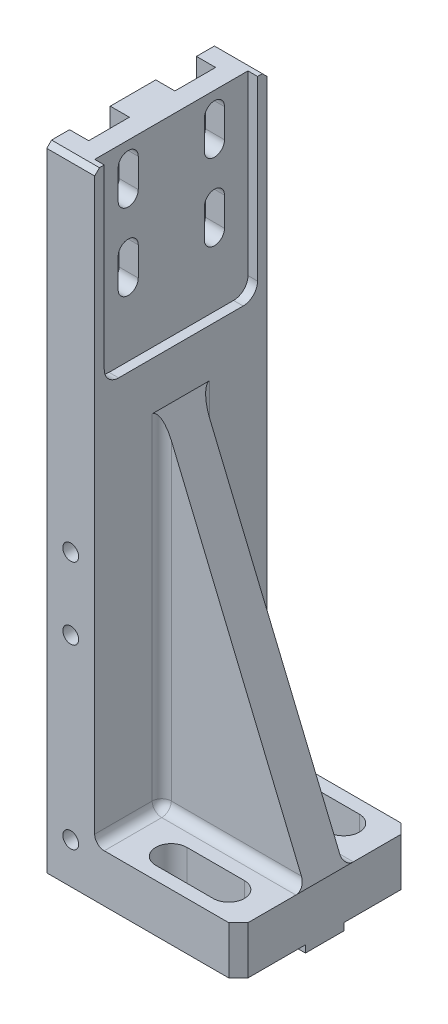
from build123d import *

# Parameters (mm, degrees)
SKETCH1_W             = 40
SKETCH1_H             = 132
BOSS_EXTRUDE1_DEPTH   = 18
SKETCH2_W             = 30
SKETCH2_H             = 122
CUT_EXTRUDE1_DEPTH    = 78.794601355
RIB2_REACH            = 73.274
SKETCH3_WALL_W        = 222.54823745
SKETCH3_WALL_H        = 8
FILLET1_R             = 2
CUT_EXTRUDE2_DEPTH    = 2
CUT_EXTRUDE3_DEPTH    = 80.246451025
CUT_EXTRUDE4_DEPTH    = 4
SKETCH9_W             = 40
SKETCH9_H             = 8
BOSS_EXTRUDE2_DEPTH   = 1.5
CUT_EXTRUDE5_DEPTH    = 135.714512952
CHAMFER1_SIZE         = 1
CHAMFER2_SIZE         = 2
M3_TAPPED_HOLE2_D     = 2.5
M3_TAPPED_HOLE2_DEPTH = 7.5
M3_TAPPED_HOLE2_TIP   = 0.751075774
M4_TAPPED_HOLE2_D     = 3.3
M4_TAPPED_HOLE2_DEPTH = 11.5
M4_TAPPED_HOLE2_TIP   = 0.991420021


with BuildPart() as part:
    # Sketch1 → Boss-Extrude1 (new, symmetric)
    with BuildSketch(Plane.XY):
        Rectangle(SKETCH1_W, SKETCH1_H)
    extrude(amount=BOSS_EXTRUDE1_DEPTH, both=True)

    # Sketch2 → Cut-Extrude1 (cut, through all)
    with BuildSketch(Plane.XY.offset(18)):
        with Locations((5, 5)):
            Rectangle(SKETCH2_W, SKETCH2_H)
    extrude(amount=-CUT_EXTRUDE1_DEPTH, mode=Mode.SUBTRACT)

    # Sketch3 wall → Rib2 (add, up to next)
    with BuildSketch(Plane(origin=(5, -20, 0), x_dir=(-0.384615384615, 0.923076923077, 0), z_dir=(-0.923076923077, -0.384615384615, 0)), mode=Mode.PRIVATE) as rib2_sk1:
        Rectangle(SKETCH3_WALL_W, SKETCH3_WALL_H)
    rib2_tool1 = extrude(rib2_sk1.sketch, amount=RIB2_REACH, mode=Mode.PRIVATE) - part.part
    add(rib2_tool1.solids().sort_by_distance((5, -20, 0))[0])

    # Fillet1
    fillet1_edges = [part.edges().sort_by_distance(p)[0] for p in [
        (-10, -56, -11),
        (-10, -56, 11),
        (-10, -20, -4),
        (-10, -20, 4),
        (5, -56, -4),
        (5, -56, 4),
    ]]
    fillet(fillet1_edges, radius=FILLET1_R)

    # Sketch4 → Cut-Extrude2 (cut)
    with BuildSketch(Plane(origin=(-10, 0, 0), x_dir=(0, 0, -1), z_dir=(1, 0, 0))):
        with BuildLine():
            Line((-16, 66), (16, 66))
            Line((16, 66), (16, 29))
            ThreePointArc((16, 29), (15.121320344, 26.878679656), (13, 26))
            Line((13, 26), (-13, 26))
            ThreePointArc((-13, 26), (-15.121320344, 26.878679656), (-16, 29))
            Line((-16, 29), (-16, 66))
        make_face()
    extrude(amount=-CUT_EXTRUDE2_DEPTH, mode=Mode.SUBTRACT)

    # Sketch5 → Cut-Extrude3 (cut, through all)
    with BuildSketch(Plane.ZY.offset(20)):
        with BuildLine():
            Line((-6.9, 62), (-6.9, 56))
            ThreePointArc((-6.9, 56), (-9, 53.9), (-11.1, 56))
            Line((-11.1, 56), (-11.1, 62))
            ThreePointArc((-11.1, 62), (-9, 64.1), (-6.9, 62))
        make_face()
        with BuildLine():
            Line((11.1, 62), (11.1, 56))
            ThreePointArc((11.1, 56), (9, 53.9), (6.9, 56))
            Line((6.9, 56), (6.9, 62))
            ThreePointArc((6.9, 62), (9, 64.1), (11.1, 62))
        make_face()
        with BuildLine():
            Line((11.1, 46), (11.1, 40))
            ThreePointArc((11.1, 40), (9, 37.9), (6.9, 40))
            Line((6.9, 40), (6.9, 46))
            ThreePointArc((6.9, 46), (9, 48.1), (11.1, 46))
        make_face()
        with BuildLine():
            Line((-6.9, 46), (-6.9, 40))
            ThreePointArc((-6.9, 40), (-9, 37.9), (-11.1, 40))
            Line((-11.1, 40), (-11.1, 46))
            ThreePointArc((-11.1, 46), (-9, 48.1), (-6.9, 46))
        make_face()
    extrude(amount=-CUT_EXTRUDE3_DEPTH, mode=Mode.SUBTRACT)

    # Sketch8 → Cut-Extrude4 (cut)
    with BuildSketch(Plane.ZY.offset(20)):
        with BuildLine():
            Line((-13.25, 56), (-13.25, 66))
            ThreePointArc((-13.25, 66), (-9, 70.25), (-4.75, 66))
            Line((-4.75, 66), (-4.75, 56))
            ThreePointArc((-4.75, 56), (-9, 51.75), (-13.25, 56))
        make_face()
        with BuildLine():
            Line((4.75, 56), (4.75, 66))
            ThreePointArc((4.75, 66), (9, 70.25), (13.25, 66))
            Line((13.25, 66), (13.25, 56))
            ThreePointArc((13.25, 56), (9, 51.75), (4.75, 56))
        make_face()
        with BuildLine():
            Line((-13.25, 40), (-13.25, 46))
            ThreePointArc((-13.25, 46), (-9, 50.25), (-4.75, 46))
            Line((-4.75, 46), (-4.75, 40))
            ThreePointArc((-4.75, 40), (-9, 35.75), (-13.25, 40))
        make_face()
        with BuildLine():
            Line((13.25, 46), (13.25, 40))
            ThreePointArc((13.25, 40), (9, 35.75), (4.75, 40))
            Line((4.75, 40), (4.75, 46))
            ThreePointArc((4.75, 46), (9, 50.25), (13.25, 46))
        make_face()
    extrude(amount=-CUT_EXTRUDE4_DEPTH, mode=Mode.SUBTRACT)

    # Sketch9 → Boss-Extrude2 (add)
    with BuildSketch(Plane.XZ.offset(66)):
        Rectangle(SKETCH9_W, SKETCH9_H)
    extrude(amount=BOSS_EXTRUDE2_DEPTH)

    # Sketch10 → Cut-Extrude5 (cut, through all)
    with BuildSketch(Plane.XZ.offset(66)):
        with BuildLine():
            Line((0, 15.25), (12, 15.25))
            ThreePointArc((12, 15.25), (15.25, 12), (12, 8.75))
            Line((12, 8.75), (0, 8.75))
            ThreePointArc((0, 8.75), (-3.25, 12), (0, 15.25))
        make_face()
        with BuildLine():
            Line((0, -8.75), (12, -8.75))
            ThreePointArc((12, -8.75), (15.25, -12), (12, -15.25))
            Line((12, -15.25), (0, -15.25))
            ThreePointArc((0, -15.25), (-3.25, -12), (0, -8.75))
        make_face()
    extrude(amount=-CUT_EXTRUDE5_DEPTH, mode=Mode.SUBTRACT)

    # Chamfer1
    chamfer1_edges = [part.edges().sort_by_distance(p)[0] for p in [
        (-15, 66, -18),
        (-15, 66, 18),
    ]]
    chamfer(chamfer1_edges, length=CHAMFER1_SIZE)

    # Chamfer2
    chamfer2_edges = [part.edges().sort_by_distance(p)[0] for p in [
        (20, -61, -18),
        (20, -61, 18),
    ]]
    chamfer(chamfer2_edges, length=CHAMFER2_SIZE)

    # M3 Tapped Hole2
    with Locations(Plane.ZY.offset(20)):
        with Locations((-14, 21), (-14, -39)):
            Hole(M3_TAPPED_HOLE2_D / 2, depth=M3_TAPPED_HOLE2_DEPTH)
            with Locations((0, 0, -(M3_TAPPED_HOLE2_DEPTH + M3_TAPPED_HOLE2_TIP / 2))):  # 118° drill point
                Cone(0, M3_TAPPED_HOLE2_D / 2, M3_TAPPED_HOLE2_TIP, mode=Mode.SUBTRACT)

    # M4 Tapped Hole2
    with Locations(Plane.XY.offset(18)):
        with Locations((-15, -5.5), (-15, -20.5)):
            Hole(M4_TAPPED_HOLE2_D / 2, depth=M4_TAPPED_HOLE2_DEPTH)
            with Locations((0, 0, -(M4_TAPPED_HOLE2_DEPTH + M4_TAPPED_HOLE2_TIP / 2))):  # 118° drill point
                Cone(0, M4_TAPPED_HOLE2_D / 2, M4_TAPPED_HOLE2_TIP, mode=Mode.SUBTRACT)

    # Sketch19 → M4 Tapped Hole3 (revolve, cut)
    with BuildSketch(Plane(origin=(-15, -57.5, 18), x_dir=(0, -1, 0), z_dir=(1, 0, 0))):
        Polygon((0, 0), (0, 12.491420021), (1.65, 11.5), (1.65, 0), align=None)
    m4_tapped_hole3 = revolve(axis=Axis((-15, -57.5, 24.35), (0, 0, -1)), mode=Mode.SUBTRACT)

    # Mirror1: M4 Tapped Hole3 across plane
    add(m4_tapped_hole3.mirror(Plane.XY), mode=Mode.SUBTRACT)


solid = part.part
